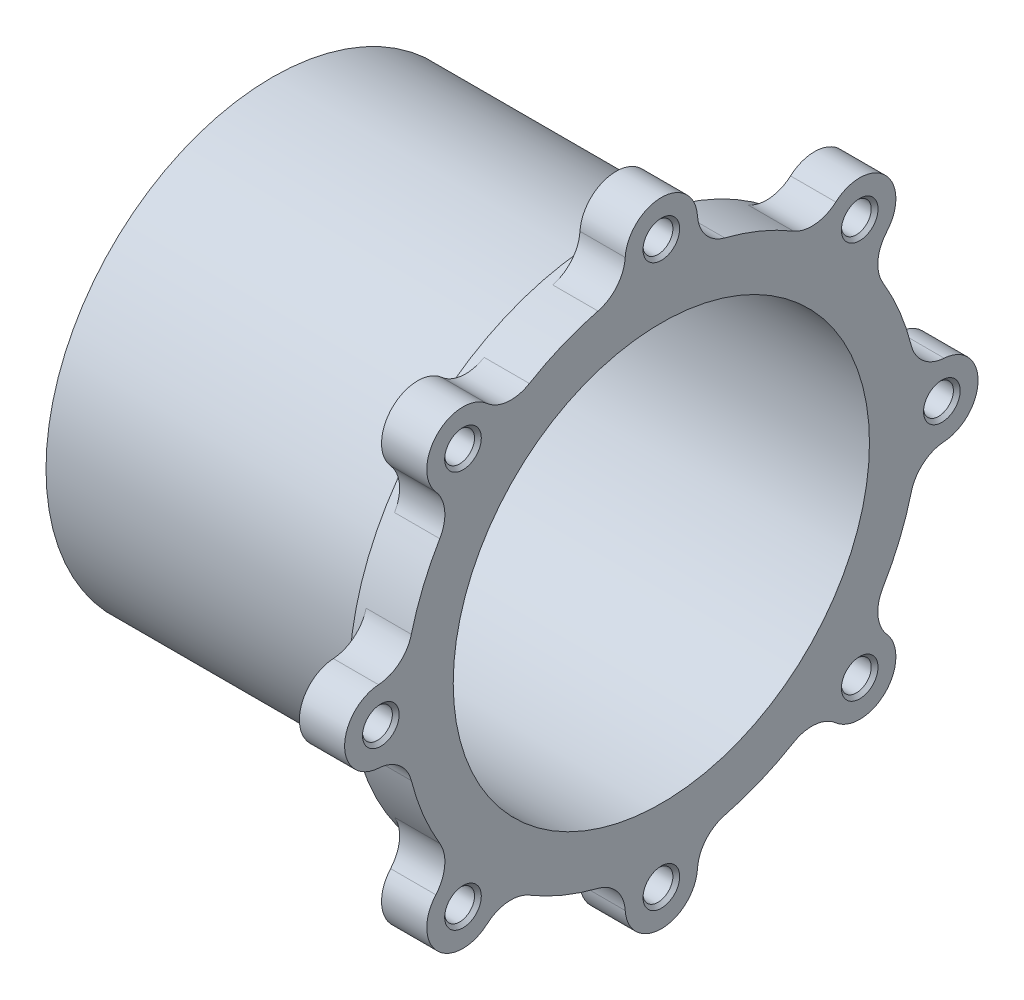
SolidWorks part; units mm, degrees
material "6061 合金"
ref_plane "前视基准面" through (0, 0, 0) normal (0, 0, 1) x (1, 0, 0)
ref_plane "上视基准面" through (0, 0, 0) normal (0, 1, 0) x (1, 0, 0)
ref_plane "右视基准面" through (0, 0, 0) normal (1, 0, 0) x (0, 0, -1)
other "Configuration Table"
sketch "草图1" plane through (0, 0, 0) normal (0, 0, 1) x (1, 0, 0)
  line L0 (-410.4784, 0) -> (20113.444, 0) construction
  line L1 (0, 13.5) -> (0, 23)
  line L2 (0, 23) -> (28, 23)
  line L3 (28, 23) -> (28, 28.5)
  line L4 (28, 28.5) -> (27, 28.5)
  line L5 (27, 28.5) -> (27, 25)
  line L6 (27, 25) -> (-10, 25)
  line L7 (-10, 25) -> (-10, 23)
  line L8 (-10, 23) -> (-3, 23)
  line L9 (-3, 23) -> (-3, 13.5)
  line L10 (-3, 13.5) -> (0, 13.5)
  dimension "D1" = 3
  dimension "D2" = 46
  dimension "D3" = 50
  dimension "D4" = 10
  dimension "D5" = 1
  dimension "D6" = 37
  dimension "D7" = 57
  dimension "D8" = 27
revolve "旋转1" add sketch "草图1" angle 360 about L0
sketch "草图2" plane through (-3, 0, 0) normal (-1, 0, 0) x (0, 0, 1)
  circle A0 centre (0, 0) radius 17.5 construction
  circle A1 centre (0, 17.5) radius 2.1
  circle A2 centre (12.3744, 12.3744) radius 2.1
  circle A3 centre (17.5, 0) radius 2.1
  circle A4 centre (12.3744, -12.3744) radius 2.1
  circle A5 centre (0, -17.5) radius 2.1
  circle A6 centre (-12.3744, -12.3744) radius 2.1
  circle A7 centre (-17.5, 0) radius 2.1
  circle A8 centre (-12.3744, 12.3744) radius 2.1
  point P22 (0, 0)
  dimension "D1" = 35
  dimension "D2" = 8
  dimension "D3" = 4.2
extrude "切除-拉伸1" cut sketch "草图2" against normal through all
sketch "草图3" plane through (28, 0, 0) normal (1, 0, 0) x (0, 0, -1)
  circle A0 centre (0, 0) radius 23 construction
  circle A1 centre (0, 0) radius 23
  circle A2 centre (0, 0) radius 35
  circle A3 centre (0, 0) radius 31.5 construction
  dimension "D1" = 70
  dimension "D2" = 63
extrude "凸台-拉伸1" add sketch "草图3" along normal blind 5
sketch "草图4" plane through (33, 0, 0) normal (1, 0, 0) x (0, 0, -1)
  circle A0 centre (0, 0) radius 31 construction
  point P3 (0, 31)
  point P7 (21.9203, 21.9203)
  point P8 (31, 0)
  point P9 (21.9203, -21.9203)
  point P10 (0, -31)
  point P11 (-21.9203, -21.9203)
  point P12 (-31, 0)
  point P13 (-21.9203, 21.9203)
  dimension "D1" = 62
  dimension "D2" = 8
hole_wizard "M4 螺纹孔1" positions "草图4" profile "草图5" tap size "M4" standard "GB" end condition through all
sketch "草图5" plane through (33, 21.9203, 21.9203) normal (0, 1, 0) x (0, 0, -1)
  line L0 (0, 0) -> (0, 43)
  line L1 (0, 43) -> (1.65, 43)
  line L2 (1.65, 43) -> (1.65, 0.375)
  line L3 (1.65, 0.375) -> (2.025, 0)
  line L5 (2.025, 0) -> (0, 0)
  line L6 (-1.65, 0.375) -> (-2.025, 0) construction
  line L11 (0, -6.35) -> (0, 107.95) construction
  dimension "通孔螺纹孔钻头直径" = 3.3
  dimension "通孔螺纹孔钻头深度" = 43
  dimension "近端锥形沉头孔直径" = 4.05
  dimension "近端锥形沉头孔角度" = 90
cosmetic thread "孔螺纹线1" parameters "D2"=4
cosmetic thread "孔螺纹线2" parameters "D2"=4
cosmetic thread "孔螺纹线3" parameters "D2"=4
cosmetic thread "孔螺纹线4" parameters "D2"=4
cosmetic thread "孔螺纹线5" parameters "D2"=4
cosmetic thread "孔螺纹线6" parameters "D2"=4
cosmetic thread "孔螺纹线7" parameters "D2"=4
cosmetic thread "孔螺纹线8" parameters "D2"=4
sketch "草图7" plane through (28, 0, 0) normal (-1, 0, 0) x (0, 0, 1)
  line L0 (0, 31) -> (0, 0) construction
  line L1 (0, 0) -> (-11.4805, 27.7164) construction
  line L2 (-16.119, 25.3017) -> (0, 0) construction
  line L3 (0, 0) -> (-6.4932, 29.2889) construction
  arc A0 (-16.119, 25.3017) -> (-6.4932, 29.2889) centre (0, 0) cw construction
  arc A1 (-6.8178, 30.7533) -> (-16.9249, 26.5668) centre (0, 0) ccw
  arc A2 (-6.1685, 27.8244) -> (-15.313, 24.0367) centre (0, 0) ccw
  arc A3 (-6.1685, 27.8244) -> (-6.8178, 30.7533) centre (-6.4932, 29.2889) ccw
  arc A4 (-16.9249, 26.5668) -> (-15.313, 24.0367) centre (-16.119, 25.3017) ccw
  arc A5 (6.4932, 29.2889) -> (16.119, 25.3017) centre (0, 0) cw construction
  arc A6 (16.9249, 26.5668) -> (6.8178, 30.7533) centre (0, 0) ccw
  arc A7 (15.313, 24.0367) -> (6.1685, 27.8244) centre (0, 0) ccw
  arc A8 (15.313, 24.0367) -> (16.9249, 26.5668) centre (16.119, 25.3017) ccw
  arc A9 (6.8178, 30.7533) -> (6.1685, 27.8244) centre (6.4932, 29.2889) ccw
  arc A10 (25.3017, 16.119) -> (29.2889, 6.4932) centre (0, 0) cw construction
  arc A11 (30.7533, 6.8178) -> (26.5668, 16.9249) centre (0, 0) ccw
  arc A12 (27.8244, 6.1685) -> (24.0367, 15.313) centre (0, 0) ccw
  arc A13 (27.8244, 6.1685) -> (30.7533, 6.8178) centre (29.2889, 6.4932) ccw
  arc A14 (26.5668, 16.9249) -> (24.0367, 15.313) centre (25.3017, 16.119) ccw
  arc A15 (29.2889, -6.4932) -> (25.3017, -16.119) centre (0, 0) cw construction
  arc A16 (26.5668, -16.9249) -> (30.7533, -6.8178) centre (0, 0) ccw
  arc A17 (24.0367, -15.313) -> (27.8244, -6.1685) centre (0, 0) ccw
  arc A18 (24.0367, -15.313) -> (26.5668, -16.9249) centre (25.3017, -16.119) ccw
  arc A19 (30.7533, -6.8178) -> (27.8244, -6.1685) centre (29.2889, -6.4932) ccw
  arc A20 (16.119, -25.3017) -> (6.4932, -29.2889) centre (0, 0) cw construction
  arc A21 (6.8178, -30.7533) -> (16.9249, -26.5668) centre (0, 0) ccw
  arc A22 (6.1685, -27.8244) -> (15.313, -24.0367) centre (0, 0) ccw
  arc A23 (6.1685, -27.8244) -> (6.8178, -30.7533) centre (6.4932, -29.2889) ccw
  arc A24 (16.9249, -26.5668) -> (15.313, -24.0367) centre (16.119, -25.3017) ccw
  arc A25 (-6.4932, -29.2889) -> (-16.119, -25.3017) centre (0, 0) cw construction
  arc A26 (-16.9249, -26.5668) -> (-6.8178, -30.7533) centre (0, 0) ccw
  arc A27 (-15.313, -24.0367) -> (-6.1685, -27.8244) centre (0, 0) ccw
  arc A28 (-15.313, -24.0367) -> (-16.9249, -26.5668) centre (-16.119, -25.3017) ccw
  arc A29 (-6.8178, -30.7533) -> (-6.1685, -27.8244) centre (-6.4932, -29.2889) ccw
  arc A30 (-25.3017, -16.119) -> (-29.2889, -6.4932) centre (0, 0) cw construction
  arc A31 (-30.7533, -6.8178) -> (-26.5668, -16.9249) centre (0, 0) ccw
  arc A32 (-27.8244, -6.1685) -> (-24.0367, -15.313) centre (0, 0) ccw
  arc A33 (-27.8244, -6.1685) -> (-30.7533, -6.8178) centre (-29.2889, -6.4932) ccw
  arc A34 (-26.5668, -16.9249) -> (-24.0367, -15.313) centre (-25.3017, -16.119) ccw
  arc A35 (-29.2889, 6.4932) -> (-25.3017, 16.119) centre (0, 0) cw construction
  arc A36 (-26.5668, 16.9249) -> (-30.7533, 6.8178) centre (0, 0) ccw
  arc A37 (-24.0367, 15.313) -> (-27.8244, 6.1685) centre (0, 0) ccw
  arc A38 (-24.0367, 15.313) -> (-26.5668, 16.9249) centre (-25.3017, 16.119) ccw
  arc A39 (-30.7533, 6.8178) -> (-27.8244, 6.1685) centre (-29.2889, 6.4932) ccw
  point P4 (-11.4805, 27.7164)
  point P19 (11.4805, 27.7164)
  point P26 (27.7164, 11.4805)
  point P33 (27.7164, -11.4805)
  point P40 (11.4805, -27.7164)
  point P47 (-11.4805, -27.7164)
  point P54 (-27.7164, -11.4805)
  point P61 (-27.7164, 11.4805)
  point P66 (0, 0)
  dimension "D1" = 22.5
  dimension "D3" = 30
  dimension "D4" = 3
  dimension "D2" = 20
  dimension "D5" = 8
extrude "切除-拉伸2" [suppressed] cut sketch "草图7" against normal through all
sketch "草图9" plane through (28, 0, 0) normal (-1, 0, 0) x (0, 0, 1)
  arc A5 (3.9921, 31.252) -> (-3.9921, 31.252) centre (0, 31) ccw
  circle A7 centre (0, 0) radius 28.5 construction
  circle A8 centre (0, 0) radius 35 construction
  arc A10 (-7.0014, 27.6266) -> (-14.5842, 24.4857) centre (0, 0) ccw
  circle A11 centre (0, 0) radius 35
  arc A12 (7.0014, 27.6266) -> (3.9921, 31.252) centre (7.9841, 31.504) cw
  arc A13 (-7.0014, 27.6266) -> (-3.9921, 31.252) centre (-7.9841, 31.504) ccw
  arc A14 (24.9213, 19.2757) -> (19.2757, 24.9213) centre (21.9203, 21.9203) ccw
  arc A15 (24.4857, 14.5842) -> (24.9213, 19.2757) centre (27.9223, 16.6311) cw
  arc A16 (14.5842, 24.4857) -> (19.2757, 24.9213) centre (16.6311, 27.9223) ccw
  arc A17 (31.252, -3.9921) -> (31.252, 3.9921) centre (31, 0) ccw
  arc A18 (27.6266, -7.0014) -> (31.252, -3.9921) centre (31.504, -7.9841) cw
  arc A19 (27.6266, 7.0014) -> (31.252, 3.9921) centre (31.504, 7.9841) ccw
  arc A20 (19.2757, -24.9213) -> (24.9213, -19.2757) centre (21.9203, -21.9203) ccw
  arc A21 (14.5842, -24.4857) -> (19.2757, -24.9213) centre (16.6311, -27.9223) cw
  arc A22 (24.4857, -14.5842) -> (24.9213, -19.2757) centre (27.9223, -16.6311) ccw
  arc A23 (-3.9921, -31.252) -> (3.9921, -31.252) centre (0, -31) ccw
  arc A24 (-7.0014, -27.6266) -> (-3.9921, -31.252) centre (-7.9841, -31.504) cw
  arc A25 (7.0014, -27.6266) -> (3.9921, -31.252) centre (7.9841, -31.504) ccw
  arc A26 (-24.9213, -19.2757) -> (-19.2757, -24.9213) centre (-21.9203, -21.9203) ccw
  arc A27 (-24.4857, -14.5842) -> (-24.9213, -19.2757) centre (-27.9223, -16.6311) cw
  arc A28 (-14.5842, -24.4857) -> (-19.2757, -24.9213) centre (-16.6311, -27.9223) ccw
  arc A29 (-31.252, 3.9921) -> (-31.252, -3.9921) centre (-31, 0) ccw
  arc A30 (-27.6266, 7.0014) -> (-31.252, 3.9921) centre (-31.504, 7.9841) cw
  arc A31 (-27.6266, -7.0014) -> (-31.252, -3.9921) centre (-31.504, -7.9841) ccw
  arc A33 (-19.2757, 24.9213) -> (-24.9213, 19.2757) centre (-21.9203, 21.9203) ccw
  arc A34 (-14.5842, 24.4857) -> (-19.2757, 24.9213) centre (-16.6311, 27.9223) cw
  arc A35 (-24.4857, 14.5842) -> (-24.9213, 19.2757) centre (-27.9223, 16.6311) ccw
  arc A36 (14.5842, 24.4857) -> (7.0014, 27.6266) centre (0, 0) ccw
  arc A37 (27.6266, 7.0014) -> (24.4857, 14.5842) centre (0, 0) ccw
  arc A38 (24.4857, -14.5842) -> (27.6266, -7.0014) centre (0, 0) ccw
  arc A39 (7.0014, -27.6266) -> (14.5842, -24.4857) centre (0, 0) ccw
  arc A40 (-14.5842, -24.4857) -> (-7.0014, -27.6266) centre (0, 0) ccw
  arc A41 (-27.6266, -7.0014) -> (-24.4857, -14.5842) centre (0, 0) ccw
  arc A42 (-24.4857, 14.5842) -> (-27.6266, 7.0014) centre (0, 0) ccw
  dimension "D1" = 8
  dimension "D2" = 4
extrude "切除-拉伸3" cut sketch "草图9" against normal blind 420
